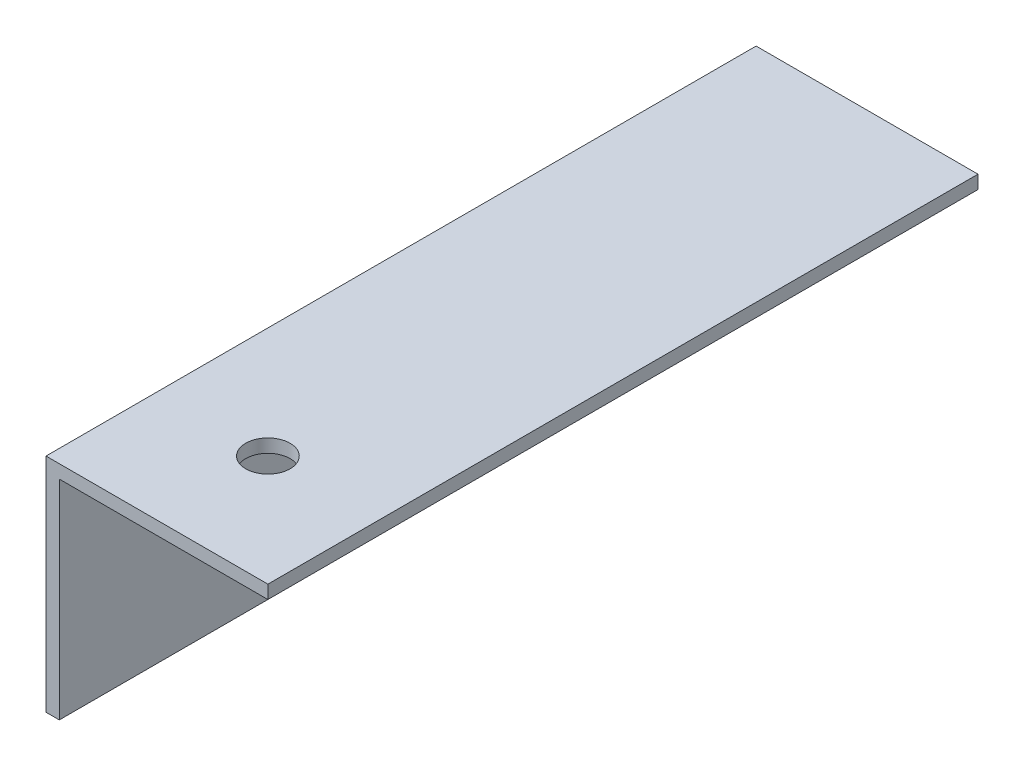
from build123d import *

# Parameters (mm, degrees)
EXTRUDE_1_DEPTH     = 160
CUT_EXTRUDE_1_DEPTH = 10


with BuildPart() as part:
    # 草图1 → 凸台-拉伸1 (new body)
    with BuildSketch(Plane.XY):
        Polygon((0, 0), (-50, 0), (-50, -50), (-47, -50), (-47, -3), (0, -3), align=None)
    extrude(amount=EXTRUDE_1_DEPTH)

    # 草图2 → 切除-拉伸1 (cut)
    with BuildSketch(Plane(origin=(0, 0, 0), x_dir=(1, 0, 0), z_dir=(0, 1, 0))):
        with BuildLine():
            ThreePointArc((-28.535533906, -131.464466094), (-28.535533906, -138.535533906), (-21.464466094, -138.535533906))
            Line((-21.464466094, -138.535533906), (-28.535533906, -131.464466094))
        make_face()
        with BuildLine():
            Line((-28.535533906, -131.464466094), (-21.464466094, -138.535533906))
            ThreePointArc((-21.464466094, -138.535533906), (-20.380602337, -136.913417162), (-20, -135))
            ThreePointArc((-20, -135), (-23.086582838, -130.380602337), (-28.535533906, -131.464466094))
        make_face()
    extrude(amount=-CUT_EXTRUDE_1_DEPTH, mode=Mode.SUBTRACT)


solid = part.part
